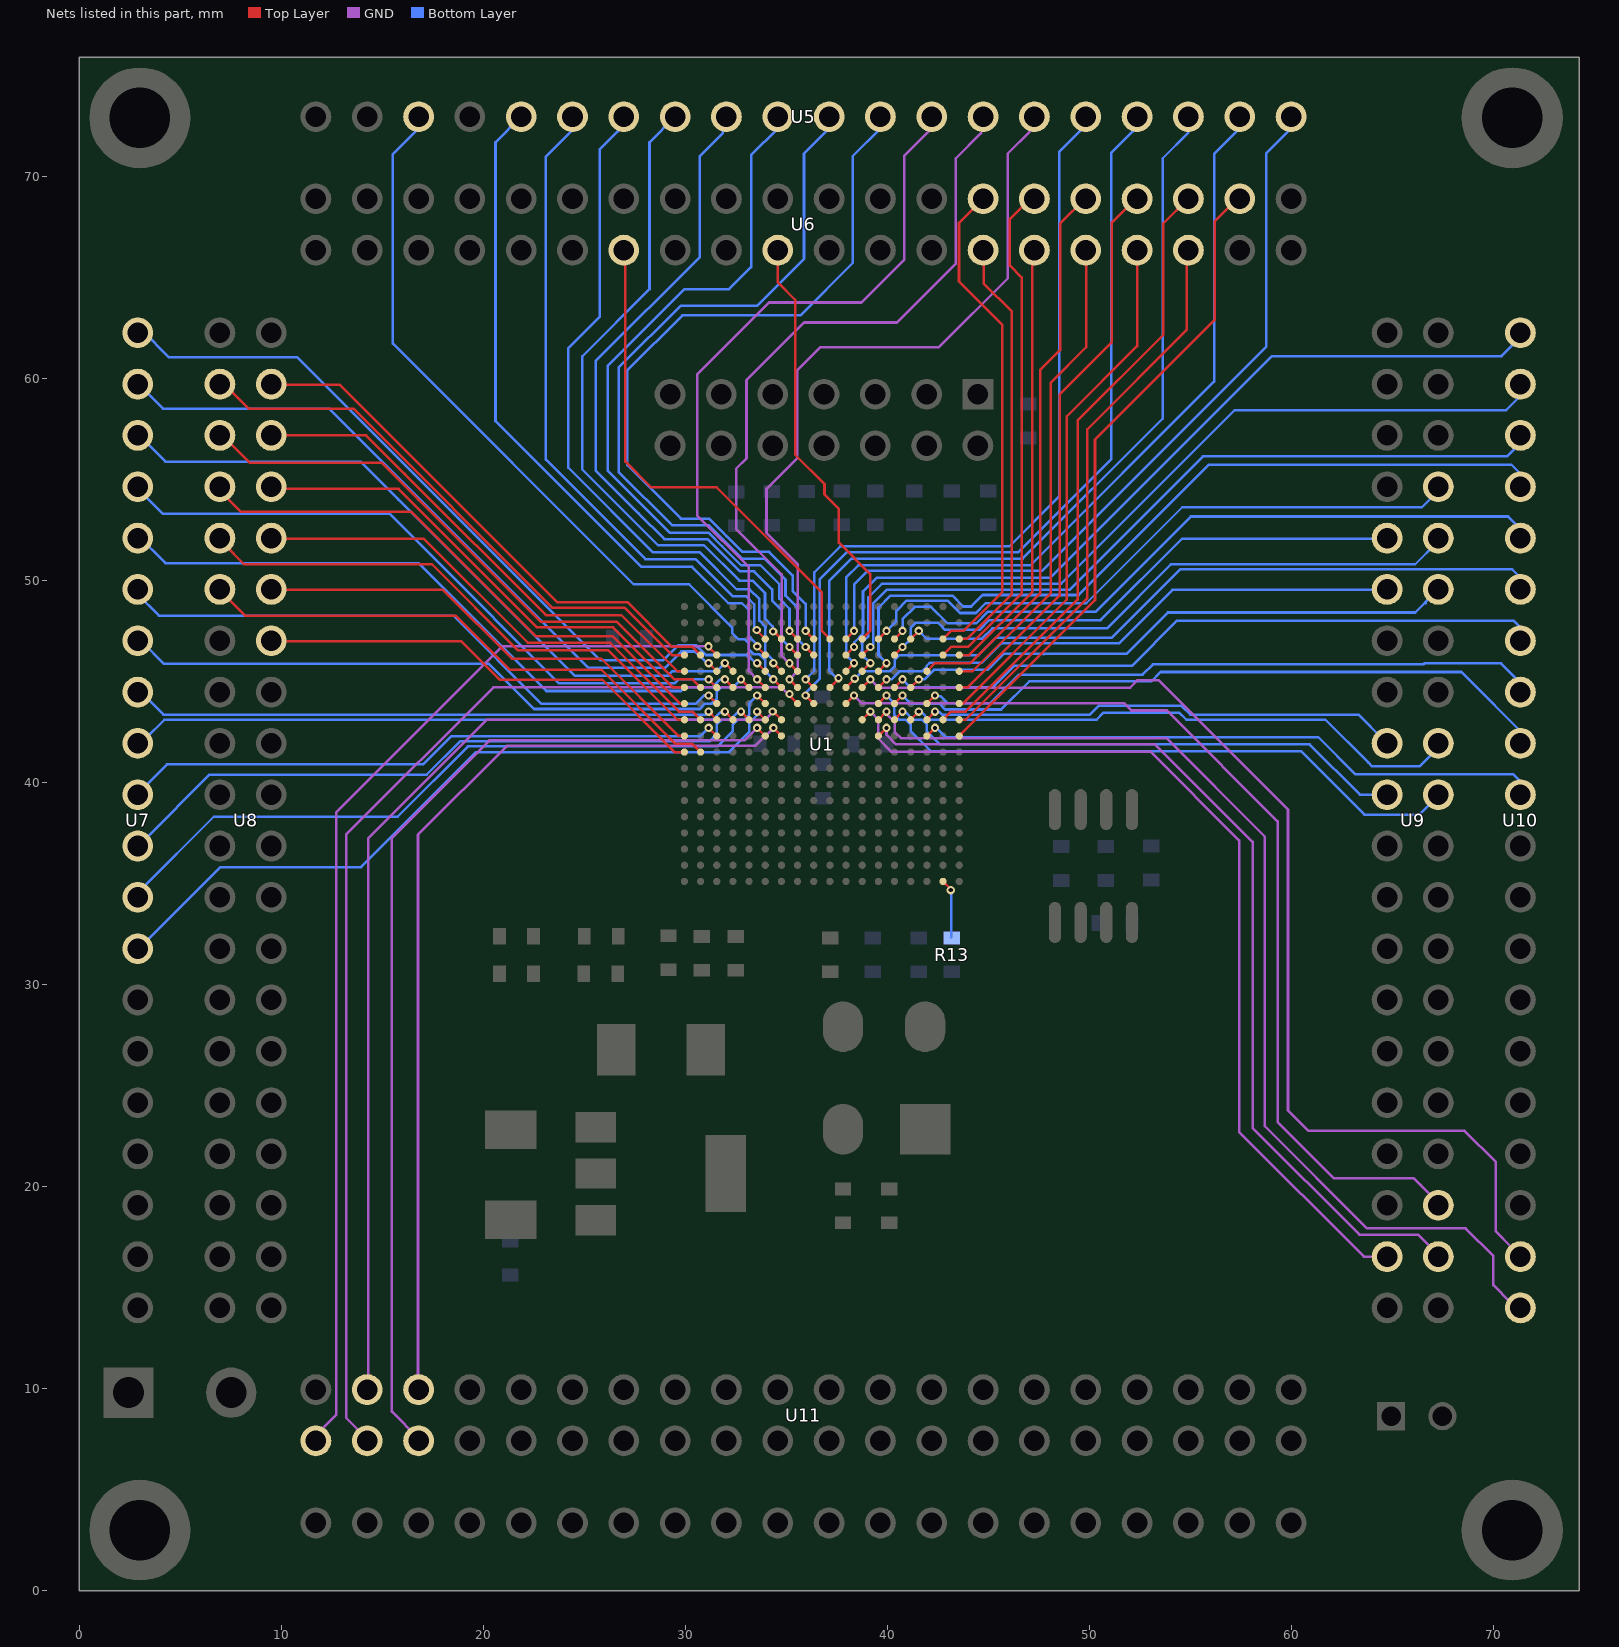
[diagram p0: the nets of this part, all layers, seen from the top]
# Altium PCB MISC103828.PcbDoc (part 2 of 4)
Units mm, origin at the board's own origin, x right, y up, seen from the top; angles counter-clockwise.
Board outline 74.24 x 75.89 mm, 4 copper layers (Top Layer, GND, POWER, Bottom Layer); 49 components, 246 nets, 670 pads, 283 vias.

## Via types
v1: diameter 0.406, hole 0.203, Top Layer to Bottom Layer, 221 vias
v2: diameter 0.61, hole 0.305, Top Layer to Bottom Layer, 43 vias
v3: diameter 0.508, hole 0.254, Top Layer to Bottom Layer, 16 vias
v4: diameter 0.432, hole 0.229, Top Layer to Bottom Layer, 3 vias

## Nets (pads, with @x,y where several pads share a name; then routed paths per layer and width w, separated by ;. In a path a pad name is that pad's centre, name@x,y a point inside that pad or via, vN(x,y) a via of type N, cw(c..) or ccw(c..) an arc to the next point about the centre after c; other vN are vias at no path point) (continued)
F_C6: U1.C6 U5.6 | length 32.6
  Top Layer w0.127: v1(33.528,47.549) v1@33.579,47.498 ; U1.C6@33.947,47.103 33.553,47.498 v1@33.579,47.498 ; v1@33.579,47.498 33.595,47.498 33.621,47.473 33.604,47.473 v1@33.579,47.498
  Bottom Layer w0.127: U5.6@24.46,72.415 24.46,72.339 23.089,70.968 23.089,55.982 28.016,51.054 30.505,51.054 32.334,49.225 32.995,49.225 33.401,48.819 33.401,47.676 v1(33.528,47.549) 33.604,47.473 v1@33.621,47.473 ; v1@33.579,47.549 33.579,47.515 v1@33.621,47.473 ; v1@33.63,47.464 v1@33.621,47.473
F_C7: U1.C7 U5.8 | length 33.5
  Top Layer w0.127: v1@34.41,47.44 U1.C7@34.747,47.103
  Bottom Layer w0.127: U5.8@29.489,72.949 28.219,71.679 28.219,64.414 24.892,61.087 24.892,55.499 28.651,51.74 30.912,51.74 32.664,49.987 33.325,49.987 33.934,49.378 33.934,48.108 34.315,47.727 v1@34.315,47.447
  other v1: 34.341,47.473
F_C8: U1.C8 U5.10 | length 35.6
  Top Layer w0.127: v1(35.147,47.503) U1.C8@35.547,47.103
  Bottom Layer w0.127: U5.10@34.569,72.365 33.249,71.044 33.249,70.968 33.249,65.507 32.156,64.414 29.947,64.414 26.162,60.63 26.162,55.423 29.235,52.349 31.156,52.349 31.816,51.689 31.819,51.689 32.759,50.749 33.706,50.749 34.646,49.809 34.646,49.098 35.147,48.596 v1(35.147,47.503)
F_C9: U1.C9 U5.12 | length 39.3
  Top Layer w0.127: v1(35.947,47.503) U1.C9@36.347,47.103
  Bottom Layer w0.127: v1(35.947,47.503) 35.947,48.838 35.306,49.479 35.306,50.241 34.138,51.41 32.817,51.41 32.029,52.197 32.027,52.197 31.915,52.309 31.915,52.311 31.166,53.061 29.769,53.061 27.127,55.702 27.127,60.401 29.845,63.119 35.687,63.119 38.278,65.71 38.278,70.993 U5.12@39.649,72.365
F_C10: U1.C10 U6.13 | length 25.1
  Top Layer w0.127: U6.13@26.975,66.091 27.026,66.04 27.026,55.88 28.296,54.61 31.547,54.61 36.751,49.405 36.751,47.499 U1.C10@37.147,47.103
F_C11: U1.C11 U5.20 | length 39.4
  Top Layer w0.127: U1.C11@37.947,47.103 v1(38.347,47.503)
  Bottom Layer w0.127: v1(38.347,47.503) 38.347,49.803 39.014,50.47 47.65,50.47 58.75,61.57 58.75,71.145 U5.20@59.969,72.365
F_C12: U1.C12 U6.19 | length 21.3
  Top Layer w0.127: U6.19@34.569,66.345 34.569,64.745 35.433,63.881 35.433,56.21 36.881,54.762 36.881,54.254 37.592,53.543 37.592,51.867 39.143,50.316 39.143,48.539 39.141,48.538 39.141,48.071 39.143,48.069 39.143,47.499 U1.C12@38.747,47.103
F_C13: U1.C13 U9.8 | length 31.6
  Top Layer w0.127: U1.C13@39.547,47.103 v1(39.947,47.503)
  Bottom Layer w0.127: v1(39.947,47.503) 40.437,47.993 40.437,48.489 40.945,48.997 42.975,48.997 43.381,48.59 43.383,48.59 43.586,48.387 44.374,48.387 44.856,48.87 49.835,48.87 54.585,53.619 66.446,53.619 U9.8@67.31,54.483
F_C14: U1.C14 U10.5 | length 35
  Top Layer w0.127: U1.C14@40.347,47.103 v1(40.747,47.503)
  Bottom Layer w0.127: v1(40.747,47.503) 40.747,48.088 41.354,48.695 42.161,48.695 42.977,47.879 44.399,47.879 44.958,48.438 50.292,48.438 55.016,53.162 70.714,53.162 U10.5@71.526,52.349
F_C15: U1.C15 U9.10 | length 28.6
  Top Layer w0.127: U1.C15@41.147,47.103 v1(41.547,47.503)
  Bottom Layer w0.127: v1(41.547,47.503) 41.941,47.11 42.51,47.11 42.518,47.117 44.679,47.117 45.187,47.625 50.851,47.625 54.026,50.8 66.116,50.8 U9.10@67.183,51.867 ; U9.10@67.208,51.841 67.259,51.892 U9.10@67.259,52.095
F_C17: U1.C17 U6.28 | length 24.7
  Top Layer w0.127: U1.C17@42.747,47.103 43.143,47.499 43.765,47.499 45.669,49.403 45.669,62.662 43.536,64.795 43.536,67.691 U6.28@44.729,68.885
F_C18: U1.C18 U6.27 | length 20.9
  Top Layer w0.127: U1.C18@43.547,47.103 43.928,47.103 46.152,49.327 46.152,63.297 44.755,64.694 44.755,65.964 U6.27@44.856,66.065
F_D1: U1.D1 U8.3 | length 28.2
  Top Layer w0.127: U8.3@7.29,59.588 8.382,58.496 13.564,58.496 23.419,48.641 27,48.641 29.338,46.303 U1.D1@29.947,46.303
F_D2: U1.D2 U8.4 | length 26.8
  Top Layer w0.127: U8.4@9.474,59.69 12.878,59.69 23.647,48.92 27.127,48.92 29.34,46.707 30.343,46.707 U1.D2@30.747,46.303
F_D3: U1.D3 U11.1 | length 53.7
  Top Layer w0.127: v1(31.14,46.736) 31.166,46.736 31.166,46.685 U1.D3@31.547,46.303
  GND w0.127: U11.1@11.709,7.722 11.735,7.722 12.725,8.712 12.725,38.532 20.93,46.736 v1(31.14,46.736)
F_D6: U1.D6 U5.5 | length 34.6
  Top Layer w0.127: v1@33.534,46.717 U1.D6@33.947,46.303
  Bottom Layer w0.127: U5.5@21.869,72.949 20.599,71.679 20.599,57.887 27.813,50.673 30.328,50.673 32.131,48.87 32.791,48.87 33.134,48.527 33.134,47.232 33.604,46.763 v1@33.604,46.685
  other v1: 33.553,46.736
F_D8: U1.D8 U5.9 | length 34.4
  Top Layer w0.127: v1(35.147,46.703) U1.D8@35.547,46.303
  Bottom Layer w0.127: U5.9@31.852,72.263 31.852,72.136 30.709,70.993 30.709,66.015 25.552,60.858 25.552,55.448 27.686,53.315 28.956,52.045 31.101,52.045 32.702,50.444 33.401,50.444 34.29,49.555 34.29,48.997 34.76,48.527 34.76,48.122 34.747,48.11 34.747,47.104 v1(35.147,46.703)
F_D9: U1.D9 U5.11 | length 38.3
  Top Layer w0.127: v1(35.947,46.703) U1.D9@36.347,46.303
  Bottom Layer w0.127: v1(35.947,46.703) 35.541,47.11 35.541,48.66 34.95,49.251 34.95,50.038 33.909,51.079 32.788,51.079 31.924,51.943 31.921,51.943 31.134,52.73 29.337,52.73 26.695,55.372 26.695,60.528 29.769,63.602 33.553,63.602 35.865,65.913 35.865,71.12 U5.11@37.109,72.365
F_D11: U1.D11 U10.1 | length 42
  Top Layer w0.127: U1.D11@37.947,46.303 v1(38.347,46.703)
  Bottom Layer w0.127: v1(38.347,46.703) 38.347,46.947 ; 38.354,46.939 38.786,47.371 38.786,49.454 39.472,50.14 48.057,50.14 59.004,61.087 70.383,61.087 ; 70.383,61.112 71.526,62.255 U10.1@71.78,62.255 ; U10.1@71.819,62.217 71.907,62.306 U10.1@71.907,62.382
F_D12: U1.D12 U10.3 | length 38.8
  Top Layer w0.127: U1.D12@38.747,46.303 v1(39.147,46.703)
  Bottom Layer w0.127: v1(39.147,46.703) 39.3,46.856 39.3,48.875 39.954,49.53 48.997,49.53 55.601,56.134 70.663,56.134 71.704,57.175 U10.3@71.78,57.175 ; U10.3@71.806,57.175 U10.3@71.806,57.302
F_D14: U1.D14 U9.9 | length 27.2
  Top Layer w0.127: U1.D14@40.347,46.303 v1(40.747,46.703)
  Bottom Layer w0.127: v1(40.747,46.703) 41.154,47.11 41.154,47.666 41.384,47.897 42.51,47.897 42.741,47.666 42.741,47.65 42.843,47.549 44.552,47.549 45.034,48.031 50.546,48.031 54.585,52.07 U9.9@64.491,52.07
F_D17: U1.D17 U6.30 | length 25.6
  Top Layer w0.127: U1.D17@42.747,46.303 43.151,46.707 43.99,46.707 46.634,49.352 46.634,64.999 46.05,65.583 46.05,67.894 47.117,68.961 U6.30@47.269,68.961
F_D18: U1.D18 U6.29 | length 21.6
  Top Layer w0.127: U1.D18@43.547,46.303 44.043,46.303 47.168,49.428 U6.29@47.168,66.116
F_DONE: R13.2 U1.V17 | length 2.9
  Top Layer w0.127: U1.V17@42.747,35.103 43.129,34.722 v1(43.129,34.671)
  Bottom Layer w0.127: R13.2@43.155,32.334 43.155,34.595 v1@43.18,34.62
F_E1: U1.E1 U8.6 | length 25.3
  Top Layer w0.127: U8.6@9.5,57.175 14.199,57.175 16.104,55.27 16.129,55.245 23.089,48.285 26.822,48.285 29.604,45.503 U1.E1@29.947,45.503
F_E3: U1.E3 U7.2 | length 35.3
  Top Layer w0.127: v1(31.147,45.903) U1.E3@31.547,45.503
  Bottom Layer w0.127: U7.2@2.946,59.69 4.14,58.496 12.37,58.496 14.275,56.591 ; 14.199,56.667 14.275,56.591 ; v1(31.147,45.903) 31.055,45.903 30.476,46.482 29.794,46.482 28.981,45.669 25.197,45.669 14.275,56.591
F_E4: U1.E4 U7.3 | length 34.8
  Top Layer w0.127: v1(31.947,45.903) U1.E4@32.347,45.503
  Bottom Layer w0.127: U7.3@2.972,57.175 4.267,55.88 13.919,55.88 15.875,53.924 ; 15.799,54 15.875,53.924 ; 29.159,45.288 24.511,45.288 15.875,53.924 ; 29.159,45.314 29.34,45.495 30.532,45.495 30.534,45.497 31.541,45.497 v1(31.947,45.903)
F_E6: U1.E6 U7.1 | length 38.4
  Top Layer w0.127: v1(33.547,45.903) U1.E6@33.947,45.503
  Bottom Layer w0.127: U7.1@3.124,62.357 4.445,61.036 10.795,61.036 25.781,46.05 28.905,46.05 29.642,46.787 30.531,46.787 30.886,46.431 ; 30.888,46.431 30.886,46.431 ; v1(33.547,45.903) 33.47,45.903 33.064,46.31 31.008,46.31 30.886,46.431
F_E7: U1.E7 U5.7 | length 33.9
  Top Layer w0.127: v1(34.347,45.903) U1.E7@34.747,45.503
  Bottom Layer w0.127: U5.7@26.67,72.288 26.67,72.238 25.756,71.323 25.756,63.043 24.206,61.493 24.206,55.575 28.397,51.384 30.709,51.384 32.537,49.555 33.172,49.555 33.655,49.073 33.655,48.006 33.96,47.701 33.96,47.648 33.947,47.636 33.947,46.448 34.315,46.079 v1@34.315,45.898 ; v1@34.334,45.917 v1(34.347,45.903)
F_E8: U1.E8 U5.14 | length 35.6
  Top Layer w0.127: v1(35.154,45.898) 35.331,45.72 U1.E8@35.547,45.503
  GND w0.127: v1(35.154,45.898) 35.128,45.898 34.754,46.272 34.754,48.116 34.76,48.122 34.76,50.305 32.512,52.553 32.512,55.524 33.02,56.032 33.02,59.919 35.865,62.763 40.462,62.763 43.383,65.684 43.383,70.891 44.628,72.136
F_E11: U1.E11 U5.19 | length 40.3
  Top Layer w0.127: U1.E11@37.947,45.503 v1(38.347,45.903)
  Bottom Layer w0.127: v1(38.347,45.903) 37.948,46.303 37.948,50.14 38.557,50.749 47.066,50.749 56.159,59.842 56.159,71.095 U5.19@57.429,72.365 ; U5.19@57.366,72.428 U5.19@57.404,72.466
F_E12: U1.E12 U10.2 | length 45.8
  Top Layer w0.127: U1.E12@38.747,45.503 v1(39.147,45.903)
  Bottom Layer w0.127: v1(39.147,45.903) 38.735,46.316 38.735,46.534 38.741,46.54 38.741,46.866 38.735,46.873 38.735,46.914 39.046,47.224 39.046,49.155 39.726,49.835 48.59,49.835 57.175,58.42 65.888,58.42 ; 70.46,58.42 65.888,58.42 ; U10.2@71.78,59.588 70.612,58.42 65.888,58.42
F_E13: U1.E13 U10.4 | length 39.3
  Top Layer w0.127: U1.E13@39.547,45.503 v1(39.947,45.903)
  Bottom Layer w0.127: v1(39.947,45.903) 39.554,46.297 39.554,48.647 40.157,49.251 43.205,49.251 43.746,48.71 44.138,48.71 44.704,49.276 49.454,49.276 55.905,55.728 70.866,55.728 U10.4@71.653,54.94
F_E16: U1.E16 U6.32 | length 27.8
  Top Layer w0.127: U1.E16@41.947,45.503 42.351,45.907 44.104,45.907 47.549,49.352 47.549,60.401 48.539,61.392 48.539,67.666 49.809,68.936 U6.32@49.809,68.986
F_E18: U1.E18 U6.31 | length 23.5
  Top Layer w0.127: U1.E18@43.547,45.503 44.208,45.503 48.082,49.378 48.082,59.792 49.835,61.544 49.835,65.989 U6.31@49.86,66.015
F_F1: U1.F1 U8.8 | length 24.2
  Top Layer w0.127: U8.8@9.855,54.534 15.799,54.534 22.657,47.676 26.416,47.676 29.388,44.703 U1.F1@29.947,44.703
F_F2: U1.F2 U8.5 | length 28.5
  Top Layer w0.127: U8.5@7.315,56.947 8.433,55.829 14.961,55.829 16.789,54 22.835,47.955 26.594,47.955 29.45,45.099 30.352,45.099 U1.F2@30.747,44.703
F_F3: U1.F3 U7.4 | length 33.1
  Top Layer w0.127: v1(31.147,45.103) U1.F3@31.547,44.703
  Bottom Layer w0.127: U7.4@2.769,54.661 4.14,53.289 15.367,53.289 17.272,51.384 ; 17.221,51.435 17.272,51.384 ; v1(31.147,45.103) 29.66,45.103 29.464,44.907 23.749,44.907 17.272,51.384
F_F4: U1.F4 U7.5 | length 33.2
  Top Layer w0.127: v1(31.947,45.103) U1.F4@32.347,44.703
  Bottom Layer w0.127: U7.5@2.87,52.248 4.267,50.851 16.789,50.851 18.732,48.908 ; 18.694,48.946 18.732,48.908 ; v1(31.947,45.103) v1@31.929,45.085 ; v1@31.979,45.085 v1@31.929,45.085 ; 18.732,48.908 23.114,44.526 29.769,44.526 29.947,44.704 31.318,44.704 31.699,45.085 v1@31.929,45.085
F_F5: U1.F5 U7.7 | length 32.4
  Top Layer w0.127: v1(32.747,45.103) U1.F5@33.147,44.703
  Bottom Layer w0.127: U7.7@3.124,46.939 4.191,45.872 20.269,45.872 22.504,43.637 30.709,43.637 30.968,43.897 31.298,43.897 31.554,44.153 31.554,44.508 31.756,44.71 32.354,44.71 v1(32.747,45.103)
F_F6: U1.F6 U5.13 | length 36.4
  Top Layer w0.127: v1(33.547,45.103) U1.F6@33.947,44.703
  GND w0.127: v1(33.547,45.103) 33.141,45.51 33.141,47.379 33.134,47.386 33.134,47.712 33.141,47.719 33.141,50.653 30.582,53.213 30.582,60.198 34.138,63.754 38.71,63.754 40.818,65.862 40.818,70.993 U5.13@42.062,72.238
F_F7: U1.F7 U5.3 | length 38.1
  Top Layer w0.127: v1(34.347,45.103) U1.F7@34.747,44.703
  Bottom Layer w0.127: U5.3@16.789,72.365 15.519,71.095 15.519,61.722 27.432,49.809 30.175,49.809 32.309,47.676 32.309,47.398 32.61,47.097 32.91,47.097 33.141,46.866 33.141,46.592 33.39,46.342 33.665,46.342 33.941,46.066 33.941,45.51 v1(34.347,45.103)
F_F8: U1.F8 U5.15 | length 37.5
  Top Layer w0.127: v1(35.147,45.103) U1.F8@35.547,44.703
  GND w0.127: v1(35.147,45.103) 35.554,45.51 35.554,50.806 34.011,52.349 34.011,54.534 35.535,56.058 35.535,60.401 36.678,61.544 42.545,61.544 45.949,64.948 45.949,71.12 47.066,72.238 U5.15@47.066,72.39
F_F9: U1.F9 U5.16 | length 38.3
  Top Layer w0.127: v1(35.947,45.103) U1.F9@36.347,44.703
  Bottom Layer w0.127: v1(35.947,45.103) 36.373,45.529 36.373,50.394 37.668,51.689 46.025,51.689 48.489,54.153 48.489,71.196 49.581,72.288 U5.16@49.581,72.314
F_F10: U1.F10 U5.18 | length 40.5
  Top Layer w0.127: U1.F10@37.147,44.703 37.592,45.148 37.592,45.161 v1(37.567,45.161)
  Bottom Layer w0.127: v1(37.567,45.161) 37.592,45.161 37.592,45.148 37.547,45.103 37.109,45.541 37.109,49.962 38.227,51.079 46.685,51.079 53.619,58.014 53.619,70.891 54.889,72.161 U5.18@54.889,72.365
F_F11: U1.F11 U10.6 | length 36.8
  Top Layer w0.127: U1.F11@37.947,44.703 v1(38.379,45.136)
  Bottom Layer w0.127: v1(38.379,45.136) 38.754,45.51 40.125,45.51 40.354,45.738 40.354,46.066 40.589,46.302 40.589,46.304 44.501,46.304 45.364,47.168 51.105,47.168 54.483,50.546 70.917,50.546 U10.6@71.755,49.708
F_F12: U1.F12 U10.19 | length 55.1
  Top Layer w0.127: U1.F12@38.747,44.703 v1(39.147,45.103)
  GND w0.127: v1(39.147,45.103) 39.554,44.697 52.012,44.697 52.375,45.06 53.416,45.06 59.817,38.659 59.817,23.774 60.833,22.758 67.793,22.758 ; 67.97,22.758 67.793,22.758 ; U10.19@70.866,17.018 70.104,17.78 70.104,21.209 68.555,22.758 67.793,22.758
F_F13: U1.F13 U9.11 | length 27.3
  Top Layer w0.127: U1.F13@39.547,44.703 v1(39.947,45.103)
  Bottom Layer w0.127: v1(39.947,45.103) 40.191,45.103 40.584,45.497 41.698,45.497 41.941,45.74 41.941,45.776 42.088,45.923 44.653,45.923 45.618,46.888 51.46,46.888 54.102,49.53 64.821,49.53 U9.11@64.846,49.555
F_F14: U1.F14 U10.7 | length 33.4
  Top Layer w0.127: U1.F14@40.347,44.703 v1(40.747,45.103)
  Bottom Layer w0.127: v1(40.747,45.103) 41.147,44.704 45.187,44.704 46.253,45.771 52.095,45.771 54.331,48.006 70.968,48.006 U10.7@71.73,47.244
F_F15: U1.F15 U9.12 | length 28.2
  Top Layer w0.127: U1.F15@41.147,44.703 v1(41.547,45.103)
  Bottom Layer w0.127: v1(41.547,45.103) 41.827,45.103 42.291,45.568 44.958,45.568 45.771,46.38 47.701,46.38 ; 47.727,46.355 47.701,46.38 ; 66.586,48.882 66.116,48.412 53.873,48.412 51.841,46.38 47.701,46.38 ; 66.624,48.87 66.624,48.92 U9.12@67.259,49.555
F_F18: U1.F18 U6.34 | length 28.1
  Top Layer w0.127: U1.F18@43.547,44.703 43.967,44.703 48.514,49.251 48.514,59.207 51.105,61.798 51.105,67.716 52.273,68.885 U6.34@52.273,68.961
F_G1: U1.G1 U8.7 | length 27.1
  Top Layer w0.127: U8.7@7.137,54.254 8.001,53.391 16.434,53.391 22.581,47.244 26.391,47.244 29.731,43.903 U1.G1@29.947,43.903
F_G3: U1.G3 U7.6 | length 31.3
  Top Layer w0.127: v1(31.147,44.303) U1.G3@31.547,43.903
  Bottom Layer w0.127: U7.6@2.845,49.352 3.937,48.26 18.517,48.26 22.885,43.891 30.505,43.891 30.918,44.303 v1(31.147,44.303)
F_G6: U1.G6 U7.12 | length 35.6
  Top Layer w0.127: v1(33.547,44.303) U1.G6@33.947,43.903
  Bottom Layer w0.127: U7.12@3.048,34.696 6.655,38.303 15.748,38.303 19.228,41.783 31.584,41.783 32.341,42.54 32.341,42.854 32.385,42.898 32.385,42.901 32.388,42.901 32.584,43.097 32.886,43.097 32.899,43.11 32.91,43.11 33.147,43.346 33.147,43.903 v1(33.547,44.303)
F_G8: U1.G8 U11.3 | length 56.4
  Top Layer w0.127: v1(35.147,44.382) 35.147,44.418 35.154,44.418 35.154,44.31 35.147,44.303 U1.G8@35.547,43.903
  GND w0.127: U11.3@14.249,7.417 14.249,7.518 13.208,8.56 13.208,37.414 20.498,44.704 34.747,44.704 35.147,44.303 35.154,44.31 35.154,44.418 35.147,44.418 v1(35.147,44.382)
F_G9: U1.G9 U5.17 | length 40.2
  Top Layer w0.127: v1(35.947,44.303) U1.G9@36.347,43.903
  Bottom Layer w0.127: v1(35.947,44.303) 35.947,44.431 36.652,45.136 36.652,50.063 37.973,51.384 46.457,51.384 51.079,56.007 51.079,71.171 U5.17@52.146,72.238
F_G11: U1.G11 U9.36 | length 48.9
  Top Layer w0.127: U1.G11@37.947,43.903 v1(38.347,44.303)
  GND w0.127: v1(38.347,44.303) 38.741,43.91 51.721,43.91 52.07,43.561 53.823,43.561 59.309,38.075 59.309,23.19 62.078,20.422 66.04,20.422 66.383,20.079 ; 66.446,20.015 66.383,20.079 ; U9.36@67.208,18.974 67.208,19.253 66.383,20.079
F_G13: U1.G13 U9.20 | length 31.2
  Top Layer w0.127: U1.G13@39.547,43.903 v1(39.947,44.303)
  Bottom Layer w0.127: v1(39.947,44.303) 40.335,43.916 40.335,43.672 40.341,43.666 40.341,43.352 40.596,43.097 40.91,43.097 41.141,42.866 41.141,42.552 42.139,41.554 60.452,41.554 63.602,38.405 66.319,38.405 U9.20@67.259,39.345
F_G14: U1.G14 U10.9 | length 34
  Top Layer w0.127: U1.G14@40.347,43.903 v1(40.747,44.303)
  Bottom Layer w0.127: v1(40.747,44.303) 41.16,43.891 41.378,43.891 41.384,43.897 42.565,43.897 42.85,43.612 45.618,43.612 47.015,45.009 53.061,45.009 53.518,45.466 68.402,45.466 U10.9@71.73,42.139
F_G16: U1.G16 U10.8 | length 31.6
  Top Layer w0.127: U1.G16@41.947,43.903 v1(42.347,44.303)
  Bottom Layer w0.127: v1(42.347,44.303) 42.379,44.272 42.622,44.272 42.984,43.91 45.078,43.91 46.507,45.339 52.629,45.339 53.137,45.847 66.523,45.847 66.573,45.898 70.358,45.898 U10.8@71.78,44.475
F_G18: U1.G18 U6.33 | length 26.2
  Top Layer w0.127: U1.G18@43.547,43.903 43.726,43.903 48.87,49.047 48.87,58.115 52.349,61.595 U6.33@52.349,66.345
F_H1: U1.H1 U8.9 | length 26.4
  Top Layer w0.127: U8.9@7.188,51.816 7.188,51.765 8.153,50.8 17.45,50.8 21.717,46.533 26.187,46.533 29.617,43.103 U1.H1@29.947,43.103
F_H2: U1.H2 U8.10 | length 24.9
  Top Layer w0.127: U8.10@9.55,52.121 9.601,52.07 17.043,52.07 22.2,46.914 26.264,46.914 29.67,43.507 30.343,43.507 U1.H2@30.747,43.103
F_H3: U1.H3 U7.8 | length 28.9
  Top Layer w0.127: v1(31.147,43.503) U1.H3@31.547,43.103
  Bottom Layer w0.127: U7.8@3.251,44.272 4.166,43.358 31.002,43.358 v1(31.147,43.503)
F_H4: U1.H4 U7.9 | length 29.8
  Top Layer w0.127: v1(31.947,43.503) U1.H4@32.347,43.103
  Bottom Layer w0.127: U7.9@3.302,42.189 4.216,43.104 31.344,43.104 31.699,43.459 v1@31.903,43.459 ; v1@31.928,43.459 v1@31.903,43.459 ; v1(31.947,43.503) v1@31.903,43.459
F_H5: U1.H5 U7.11 | length 33.1
  Top Layer w0.127: v1(32.747,43.503) U1.H5@33.147,43.103
  Bottom Layer w0.127: U7.11@3.2,37.135 6.452,40.386 17.196,40.386 18.847,42.037 19.533,42.037 ; 19.456,42.037 19.533,42.037 ; v1(32.747,43.503) 32.629,43.503 32.235,43.11 31.797,43.11 31.547,42.86 31.547,42.393 31.191,42.037 19.533,42.037
F_H6: U1.H6 U7.13 | length 36.1
  Top Layer w0.127: v1(33.547,43.503) U1.H6@33.947,43.103
  Bottom Layer w0.127: U7.13@3.15,31.953 3.15,31.979 6.985,35.814 13.945,35.814 19.634,41.504 32.156,41.504 33.147,42.494 33.147,42.926 33.547,43.326 v1(33.547,43.503)
F_H7: U1.H7 U11.4 | length 50.5
  Top Layer w0.127: v1(34.315,43.51) 34.341,43.51 U1.H7@34.747,43.103
  GND w0.127: 14.3,11.582 14.3,11.684 ; U11.4@14.326,10.084 14.3,10.109 14.3,11.684 ; v1(34.315,43.51) 34.341,43.51 34.347,43.503 33.954,43.11 20.173,43.11 14.3,37.236 14.3,11.684
F_H12: U1.H12 U9.37 | length 46.3
  Top Layer w0.127: U1.H12@38.747,43.103 v1(39.147,43.503)
  GND w0.127: v1(39.147,43.503) 39.548,43.103 39.548,42.164 40.183,41.529 53.01,41.529 57.404,37.135 57.404,22.708 63.576,16.535 U9.37@64.719,16.535
F_H13: U1.H13 U10.20 | length 53.2
  Top Layer w0.127: U1.H13@39.547,43.103 v1(39.947,43.503)
  GND w0.127: v1(39.947,43.503) 39.947,43.387 40.347,42.988 40.347,42.508 40.665,42.189 53.797,42.189 58.674,37.313 58.674,22.987 63.729,17.932 67.996,17.932 ; 68.097,17.932 67.996,17.932 ; U10.20@70.828,14.275 69.977,15.126 69.977,16.561 68.605,17.932 67.996,17.932
F_H14: U1.H14 U9.19 | length 26.4
  Top Layer w0.127: U1.H14@40.347,43.103 v1(40.747,43.503)
  Bottom Layer w0.127: v1(40.747,43.503) 40.863,43.503 41.263,43.104 41.704,43.104 41.941,42.866 41.941,42.539 42.596,41.885 60.198,41.885 60.249,41.885 60.884,41.885 63.373,39.395 U9.19@64.719,39.395
F_H15: U1.H15 U9.18 | length 28.3
  Top Layer w0.127: U1.H15@41.147,43.103 v1(41.547,43.503)
  Bottom Layer w0.127: v1@41.529,43.561 v1@41.587,43.503 ; v1(41.547,43.503) v1@41.587,43.503 ; U9.18@67.183,41.656 66.319,40.792 63.983,40.792 63.792,40.983 61.671,43.104 54.788,43.104 54.432,43.459 50.698,43.459 50.343,43.104 42.063,43.104 41.663,43.503 v1@41.587,43.503 ; U9.18@67.234,41.605 U9.18@67.437,41.808
F_H16: U1.H16 U9.17 | length 23.7
  Top Layer w0.127: U1.H16@41.947,43.103 v1(42.347,43.503)
  Bottom Layer w0.127: v1(42.347,43.503) 42.526,43.503 42.545,43.485 42.57,43.485 42.697,43.358 50.013,43.358 50.444,43.79 54.559,43.79 54.991,43.358 63.297,43.358 U9.17@64.541,42.113
F_H17: U1.H17 U6.36 | length 31.3
  Top Layer w0.127: U1.H17@42.747,43.103 43.151,43.507 43.863,43.507 49.403,49.047 49.403,57.912 53.645,62.154 53.645,67.666 54.838,68.859 U6.36@54.838,68.936
F_H18: U1.H18 U6.35 | length 27.9
  Top Layer w0.127: U1.H18@43.547,43.103 43.865,43.103 49.886,49.124 49.886,57.48 54.813,62.408 54.813,66.091 U6.35@54.788,66.116
F_J1: U1.J1 U8.12 | length 23.4
  Top Layer w0.127: U8.12@9.525,49.505 9.55,49.53 18.009,49.53 21.412,46.126 25.832,46.126 29.655,42.303 U1.J1@29.947,42.303
F_J3: U1.J3 U7.10 | length 29.9
  Top Layer w0.127: v1(31.147,42.703) U1.J3@31.547,42.303
  Bottom Layer w0.127: U7.10@3.099,39.649 4.343,40.894 17.018,40.894 18.415,42.291 30.735,42.291 v1(31.147,42.703)
F_J6: U1.J6 U11.5 | length 51.3
  Top Layer w0.127: v1(33.547,42.703) U1.J6@33.947,42.303
  GND w0.127: U11.5@16.789,7.417 16.789,7.544 15.469,8.865 15.469,37.262 20.295,42.088 32.932,42.088 v1(33.547,42.703)
F_J7: U1.J7 U11.6 | length 47.8
  Top Layer w0.127: v1(34.347,42.703) U1.J7@34.747,42.303
  GND w0.127: U11.6@16.789,9.957 16.764,9.982 16.764,37.414 21.158,41.808 33.452,41.808 v1(34.347,42.703)
F_J13: U1.J13 U9.38 | length 47.2
  Top Layer w0.127: U1.J13@39.547,42.303 v1(39.947,42.703)
  GND w0.127: v1(39.947,42.703) 39.947,42.367 40.43,41.885 53.238,41.885 58.064,37.059 58.064,22.911 63.348,17.628 66.243,17.628 U9.38@67.259,16.612
F_J16: U1.J16 U10.10 | length 31
  Top Layer w0.127: U1.J16@41.947,42.303 v1(42.347,42.703)
  Bottom Layer w0.127: v1(42.347,42.703) 42.412,42.703 42.875,42.24 61.316,42.24 63.144,40.411 70.942,40.411 U10.10@71.603,39.751
F_J18: U1.J18 U6.38 | length 32.5
  Top Layer w0.127: U1.J18@43.547,42.303 50.267,49.023 50.267,56.972 56.185,62.89 56.185,67.767 U6.38@57.455,69.037
F_K1: U1.K1 U8.14 | length 22.4
  Top Layer w0.127: U8.14@9.779,46.99 18.898,46.99 20.803,45.085 25.883,45.085 29.464,41.503 U1.K1@29.947,41.503
F_K2: U1.K2 U8.11 | length 27
  Top Layer w0.127: U8.11@7.036,49.428 8.204,48.26 18.618,48.26 21.311,45.568 25.857,45.568 29.517,41.907 30.343,41.907 U1.K2@30.747,41.503